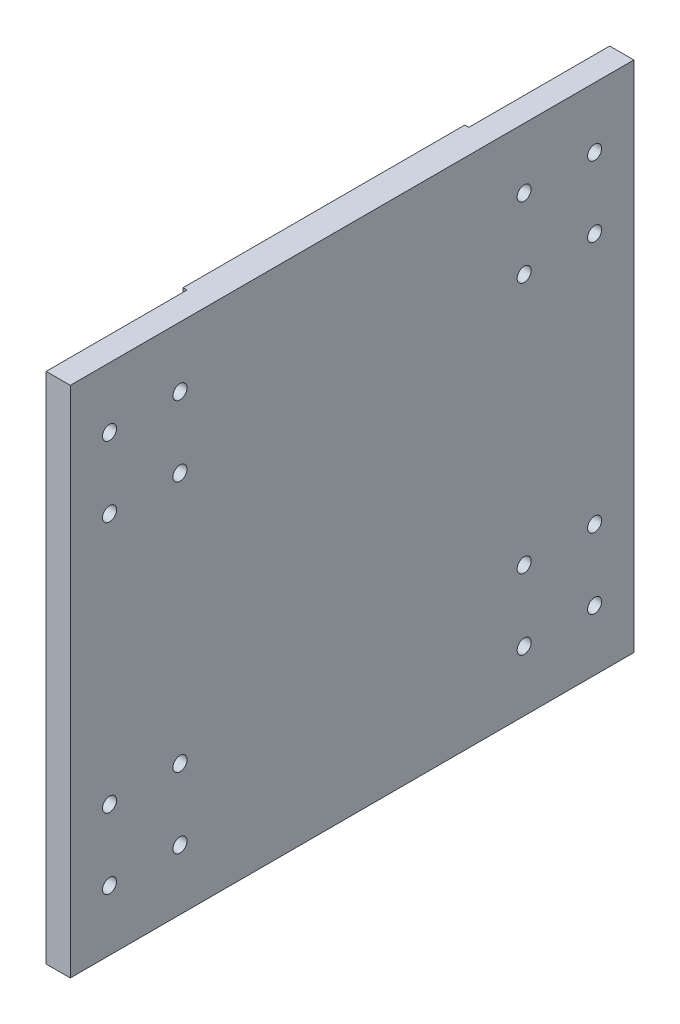
from build123d import *

# Parameters (mm, degrees)
SKETCH1_W           = 280
SKETCH1_H           = 255
SKETCH1_R           = 3.5
BOSS_EXTRUDE1_DEPTH = 14
SKETCH6_W           = 70
SKETCH6_H           = 255
CUT_EXTRUDE3_DEPTH  = 2


with BuildPart() as part:
    # Sketch1 → Boss-Extrude1 (new body)
    with BuildSketch(Plane(origin=(0, 0, 0), x_dir=(0, 0, -1), z_dir=(1, 0, 0))):
        Rectangle(SKETCH1_W, SKETCH1_H)
        with Locations((-120.5, 97.5)):
            Circle(SKETCH1_R, mode=Mode.SUBTRACT)
        with Locations((-85.5, 97.5)):
            Circle(SKETCH1_R, mode=Mode.SUBTRACT)
        with Locations((-120.5, -97.5)):
            Circle(SKETCH1_R, mode=Mode.SUBTRACT)
        with Locations((-85.5, -97.5)):
            Circle(SKETCH1_R, mode=Mode.SUBTRACT)
        with Locations((-120.5, 62.5)):
            Circle(SKETCH1_R, mode=Mode.SUBTRACT)
        with Locations((-85.5, 62.5)):
            Circle(SKETCH1_R, mode=Mode.SUBTRACT)
        with Locations((-120.5, -62.5)):
            Circle(SKETCH1_R, mode=Mode.SUBTRACT)
        with Locations((-85.5, -62.5)):
            Circle(SKETCH1_R, mode=Mode.SUBTRACT)
        with Locations((85.5, 97.5)):
            Circle(SKETCH1_R, mode=Mode.SUBTRACT)
        with Locations((120.5, 97.5)):
            Circle(SKETCH1_R, mode=Mode.SUBTRACT)
        with Locations((85.5, -62.5)):
            Circle(SKETCH1_R, mode=Mode.SUBTRACT)
        with Locations((120.5, -62.5)):
            Circle(SKETCH1_R, mode=Mode.SUBTRACT)
        with Locations((85.5, -97.5)):
            Circle(SKETCH1_R, mode=Mode.SUBTRACT)
        with Locations((120.5, -97.5)):
            Circle(SKETCH1_R, mode=Mode.SUBTRACT)
        with Locations((85.5, 62.5)):
            Circle(SKETCH1_R, mode=Mode.SUBTRACT)
        with Locations((120.5, 62.5)):
            Circle(SKETCH1_R, mode=Mode.SUBTRACT)
    extrude(amount=BOSS_EXTRUDE1_DEPTH)

    # Sketch6 → Cut-Extrude3 (cut)
    with BuildSketch(Plane.ZY):
        with Locations((-105, 0)):
            Rectangle(SKETCH6_W, SKETCH6_H)
        with Locations((105, 0)):
            Rectangle(SKETCH6_W, SKETCH6_H)
    extrude(amount=-CUT_EXTRUDE3_DEPTH, mode=Mode.SUBTRACT)


solid = part.part
